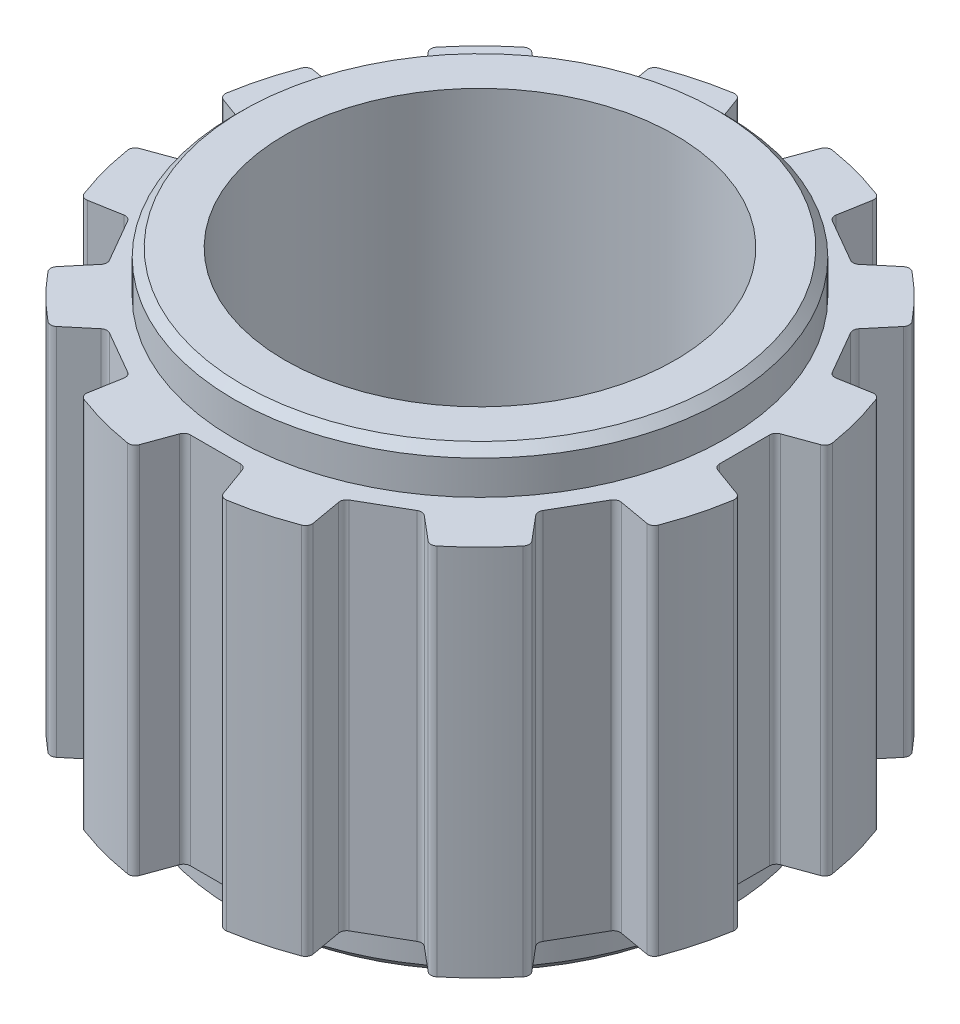
from build123d import *

# Parameters (mm, degrees)
SKETCH_1_R          = 11.5
EXTRUDE_1_DEPTH     = 27
CUT_EXTRUDE_START   = -2.5
SKETCH_2_R          = 18.1
SKETCH_2_R_2        = 14.5
CUT_EXTRUDE_1_DEPTH = 2.5
SKETCH_3_R          = 18.1
SKETCH_3_R_2        = 14.5
CUT_EXTRUDE_2_DEPTH = 2.5
CHAMFER_1_SIZE      = 0.5


with BuildPart() as part:
    # 草图1 → 拉伸1 (new body)
    with BuildSketch(Plane(origin=(0, 0, 0), x_dir=(1, 0, 0), z_dir=(0, 1, 0))):
        with BuildLine():
            Line((7.8, 13.509996299), (9.07298545, 12.775037807))
            ThreePointArc((9.07298545, 12.775037807), (9.307847747, 12.722970089), (9.530100494, 12.815030191))
            Line((9.530100494, 12.815030191), (10.949982696, 14.006452823))
            ThreePointArc((10.949982696, 14.006452823), (11.204599636, 14.100027245), (11.460365485, 14.009640357))
            ThreePointArc((11.460365485, 14.009640357), (12.798632739, 12.798632739), (14.009640357, 11.460365485))
            ThreePointArc((14.009640357, 11.460365485), (14.100027245, 11.204599636), (14.006452823, 10.949982696))
            Line((14.006452823, 10.949982696), (12.815030191, 9.530100494))
            ThreePointArc((12.815030191, 9.530100494), (12.722970089, 9.307847747), (12.775037807, 9.07298545))
            Line((12.775037807, 9.07298545), (13.509996299, 7.8))
            Line((13.509996299, 7.8), (14.244954791, 6.52701455))
            ThreePointArc((14.244954791, 6.52701455), (14.422317648, 6.364491435), (14.660824224, 6.333091449))
            Line((14.660824224, 6.333091449), (16.486189597, 6.654952614))
            ThreePointArc((16.486189597, 6.654952614), (16.753481547, 6.60868197), (16.929787826, 6.402521705))
            ThreePointArc((16.929787826, 6.402521705), (17.483257456, 4.684624716), (17.86288719, 2.920147468))
            ThreePointArc((17.86288719, 2.920147468), (17.813281606, 2.653454302), (17.604935309, 2.479736774))
            Line((17.604935309, 2.479736774), (15.863191943, 1.845794033))
            ThreePointArc((15.863191943, 1.845794033), (15.672339182, 1.699347559), (15.6, 1.469916985))
            Line((15.6, 1.469916985), (15.6, 0))
            Line((15.6, 0), (15.6, -1.469916985))
            ThreePointArc((15.6, -1.469916985), (15.672339182, -1.699347559), (15.863191943, -1.845794033))
            Line((15.863191943, -1.845794033), (17.604935309, -2.479736774))
            ThreePointArc((17.604935309, -2.479736774), (17.813281606, -2.653454302), (17.86288719, -2.920147468))
            ThreePointArc((17.86288719, -2.920147468), (17.483257456, -4.684624716), (16.929787826, -6.402521705))
            ThreePointArc((16.929787826, -6.402521705), (16.753481547, -6.60868197), (16.486189597, -6.654952614))
            Line((16.486189597, -6.654952614), (14.660824224, -6.333091449))
            ThreePointArc((14.660824224, -6.333091449), (14.422317648, -6.364491435), (14.244954791, -6.52701455))
            Line((14.244954791, -6.52701455), (13.509996299, -7.8))
            Line((13.509996299, -7.8), (12.775037807, -9.07298545))
            ThreePointArc((12.775037807, -9.07298545), (12.722970089, -9.307847747), (12.815030191, -9.530100494))
            Line((12.815030191, -9.530100494), (14.006452823, -10.949982696))
            ThreePointArc((14.006452823, -10.949982696), (14.100027245, -11.204599636), (14.009640357, -11.460365485))
            ThreePointArc((14.009640357, -11.460365485), (12.798632739, -12.798632739), (11.460365485, -14.009640357))
            ThreePointArc((11.460365485, -14.009640357), (11.204599636, -14.100027245), (10.949982696, -14.006452823))
            Line((10.949982696, -14.006452823), (9.530100494, -12.815030191))
            ThreePointArc((9.530100494, -12.815030191), (9.307847747, -12.722970089), (9.07298545, -12.775037807))
            Line((9.07298545, -12.775037807), (7.8, -13.509996299))
            Line((7.8, -13.509996299), (6.52701455, -14.244954791))
            ThreePointArc((6.52701455, -14.244954791), (6.364491435, -14.422317648), (6.333091449, -14.660824224))
            Line((6.333091449, -14.660824224), (6.654952614, -16.486189597))
            ThreePointArc((6.654952614, -16.486189597), (6.60868197, -16.753481547), (6.402521705, -16.929787826))
            ThreePointArc((6.402521705, -16.929787826), (4.684624716, -17.483257456), (2.920147468, -17.86288719))
            ThreePointArc((2.920147468, -17.86288719), (2.653454302, -17.813281606), (2.479736774, -17.604935309))
            Line((2.479736774, -17.604935309), (1.845794033, -15.863191943))
            ThreePointArc((1.845794033, -15.863191943), (1.699347559, -15.672339182), (1.469916985, -15.6))
            Line((1.469916985, -15.6), (0, -15.6))
            Line((0, -15.6), (-1.469916985, -15.6))
            ThreePointArc((-1.469916985, -15.6), (-1.699347559, -15.672339182), (-1.845794033, -15.863191943))
            Line((-1.845794033, -15.863191943), (-2.479736774, -17.604935309))
            ThreePointArc((-2.479736774, -17.604935309), (-2.653454302, -17.813281606), (-2.920147468, -17.86288719))
            ThreePointArc((-2.920147468, -17.86288719), (-4.684624716, -17.483257456), (-6.402521705, -16.929787826))
            ThreePointArc((-6.402521705, -16.929787826), (-6.60868197, -16.753481547), (-6.654952614, -16.486189597))
            Line((-6.654952614, -16.486189597), (-6.333091449, -14.660824224))
            ThreePointArc((-6.333091449, -14.660824224), (-6.364491435, -14.422317648), (-6.52701455, -14.244954791))
            Line((-6.52701455, -14.244954791), (-7.8, -13.509996299))
            Line((-7.8, -13.509996299), (-9.07298545, -12.775037807))
            ThreePointArc((-9.07298545, -12.775037807), (-9.307847747, -12.722970089), (-9.530100494, -12.815030191))
            Line((-9.530100494, -12.815030191), (-10.949982696, -14.006452823))
            ThreePointArc((-10.949982696, -14.006452823), (-11.204599636, -14.100027245), (-11.460365485, -14.009640357))
            ThreePointArc((-11.460365485, -14.009640357), (-12.798632739, -12.798632739), (-14.009640357, -11.460365485))
            ThreePointArc((-14.009640357, -11.460365485), (-14.100027245, -11.204599636), (-14.006452823, -10.949982696))
            Line((-14.006452823, -10.949982696), (-12.815030191, -9.530100494))
            ThreePointArc((-12.815030191, -9.530100494), (-12.722970089, -9.307847747), (-12.775037807, -9.07298545))
            Line((-12.775037807, -9.07298545), (-13.509996299, -7.8))
            Line((-13.509996299, -7.8), (-14.244954791, -6.52701455))
            ThreePointArc((-14.244954791, -6.52701455), (-14.422317648, -6.364491435), (-14.660824224, -6.333091449))
            Line((-14.660824224, -6.333091449), (-16.486189597, -6.654952614))
            ThreePointArc((-16.486189597, -6.654952614), (-16.753481547, -6.60868197), (-16.929787826, -6.402521705))
            ThreePointArc((-16.929787826, -6.402521705), (-17.483257456, -4.684624716), (-17.86288719, -2.920147468))
            ThreePointArc((-17.86288719, -2.920147468), (-17.813281606, -2.653454302), (-17.604935309, -2.479736774))
            Line((-17.604935309, -2.479736774), (-15.863191943, -1.845794033))
            ThreePointArc((-15.863191943, -1.845794033), (-15.672339182, -1.699347559), (-15.6, -1.469916985))
            Line((-15.6, -1.469916985), (-15.6, 0))
            Line((-15.6, 0), (-15.6, 1.469916985))
            ThreePointArc((-15.6, 1.469916985), (-15.672339182, 1.699347559), (-15.863191943, 1.845794033))
            Line((-15.863191943, 1.845794033), (-17.604935309, 2.479736774))
            ThreePointArc((-17.604935309, 2.479736774), (-17.813281606, 2.653454302), (-17.86288719, 2.920147468))
            ThreePointArc((-17.86288719, 2.920147468), (-17.483257456, 4.684624716), (-16.929787826, 6.402521705))
            ThreePointArc((-16.929787826, 6.402521705), (-16.753481547, 6.60868197), (-16.486189597, 6.654952614))
            Line((-16.486189597, 6.654952614), (-14.660824224, 6.333091449))
            ThreePointArc((-14.660824224, 6.333091449), (-14.422317648, 6.364491435), (-14.244954791, 6.52701455))
            Line((-14.244954791, 6.52701455), (-13.509996299, 7.8))
            Line((-13.509996299, 7.8), (-12.775037807, 9.07298545))
            ThreePointArc((-12.775037807, 9.07298545), (-12.722970089, 9.307847747), (-12.815030191, 9.530100494))
            Line((-12.815030191, 9.530100494), (-14.006452823, 10.949982696))
            ThreePointArc((-14.006452823, 10.949982696), (-14.100027245, 11.204599636), (-14.009640357, 11.460365485))
            ThreePointArc((-14.009640357, 11.460365485), (-12.798632739, 12.798632739), (-11.460365485, 14.009640357))
            ThreePointArc((-11.460365485, 14.009640357), (-11.204599636, 14.100027245), (-10.949982696, 14.006452823))
            Line((-10.949982696, 14.006452823), (-9.530100494, 12.815030191))
            ThreePointArc((-9.530100494, 12.815030191), (-9.307847747, 12.722970089), (-9.07298545, 12.775037807))
            Line((-9.07298545, 12.775037807), (-7.8, 13.509996299))
            Line((-7.8, 13.509996299), (-6.52701455, 14.244954791))
            ThreePointArc((-6.52701455, 14.244954791), (-6.364491435, 14.422317648), (-6.333091449, 14.660824224))
            Line((-6.333091449, 14.660824224), (-6.654952614, 16.486189597))
            ThreePointArc((-6.654952614, 16.486189597), (-6.60868197, 16.753481547), (-6.402521705, 16.929787826))
            ThreePointArc((-6.402521705, 16.929787826), (-4.684624716, 17.483257456), (-2.920147468, 17.86288719))
            ThreePointArc((-2.920147468, 17.86288719), (-2.653454302, 17.813281606), (-2.479736774, 17.604935309))
            Line((-2.479736774, 17.604935309), (-1.845794033, 15.863191943))
            ThreePointArc((-1.845794033, 15.863191943), (-1.699347559, 15.672339182), (-1.469916985, 15.6))
            Line((-1.469916985, 15.6), (0, 15.6))
            Line((0, 15.6), (1.469916985, 15.6))
            ThreePointArc((1.469916985, 15.6), (1.699347559, 15.672339182), (1.845794033, 15.863191943))
            Line((1.845794033, 15.863191943), (2.479736774, 17.604935309))
            ThreePointArc((2.479736774, 17.604935309), (2.653454302, 17.813281606), (2.920147468, 17.86288719))
            ThreePointArc((2.920147468, 17.86288719), (4.684624716, 17.483257456), (6.402521705, 16.929787826))
            ThreePointArc((6.402521705, 16.929787826), (6.60868197, 16.753481547), (6.654952614, 16.486189597))
            Line((6.654952614, 16.486189597), (6.333091449, 14.660824224))
            ThreePointArc((6.333091449, 14.660824224), (6.364491435, 14.422317648), (6.52701455, 14.244954791))
            Line((6.52701455, 14.244954791), (7.8, 13.509996299))
        make_face()
        with Locations(Location((0, 0, 0), (0, 0, 270))):
            Circle(SKETCH_1_R, mode=Mode.SUBTRACT)
    extrude(amount=EXTRUDE_1_DEPTH)

    # 草图2 → 切除-拉伸1 (cut)
    with BuildSketch(Plane(origin=(0, 27, 0), x_dir=(-1, 0, 0), z_dir=(0, 1, 0)).offset(CUT_EXTRUDE_START)):
        Circle(SKETCH_2_R)
        with Locations(Location((0, 0, 0), (0, 0, 90))):
            Circle(SKETCH_2_R_2, mode=Mode.SUBTRACT)
    extrude(amount=CUT_EXTRUDE_1_DEPTH, mode=Mode.SUBTRACT)

    # 草图3 → 切除-拉伸2 (cut)
    with BuildSketch(Plane.XZ):
        Circle(SKETCH_3_R)
        with Locations(Location((0, 0, 0), (0, 0, 90))):
            Circle(SKETCH_3_R_2, mode=Mode.SUBTRACT)
    extrude(amount=-CUT_EXTRUDE_2_DEPTH, mode=Mode.SUBTRACT)

    # 倒角1
    chamfer_1_edges = [part.edges().sort_by_distance(p)[0] for p in [
        (0, 27, -14.5),
        (0, 0, -14.5),
    ]]
    chamfer(chamfer_1_edges, length=CHAMFER_1_SIZE)


solid = part.part
